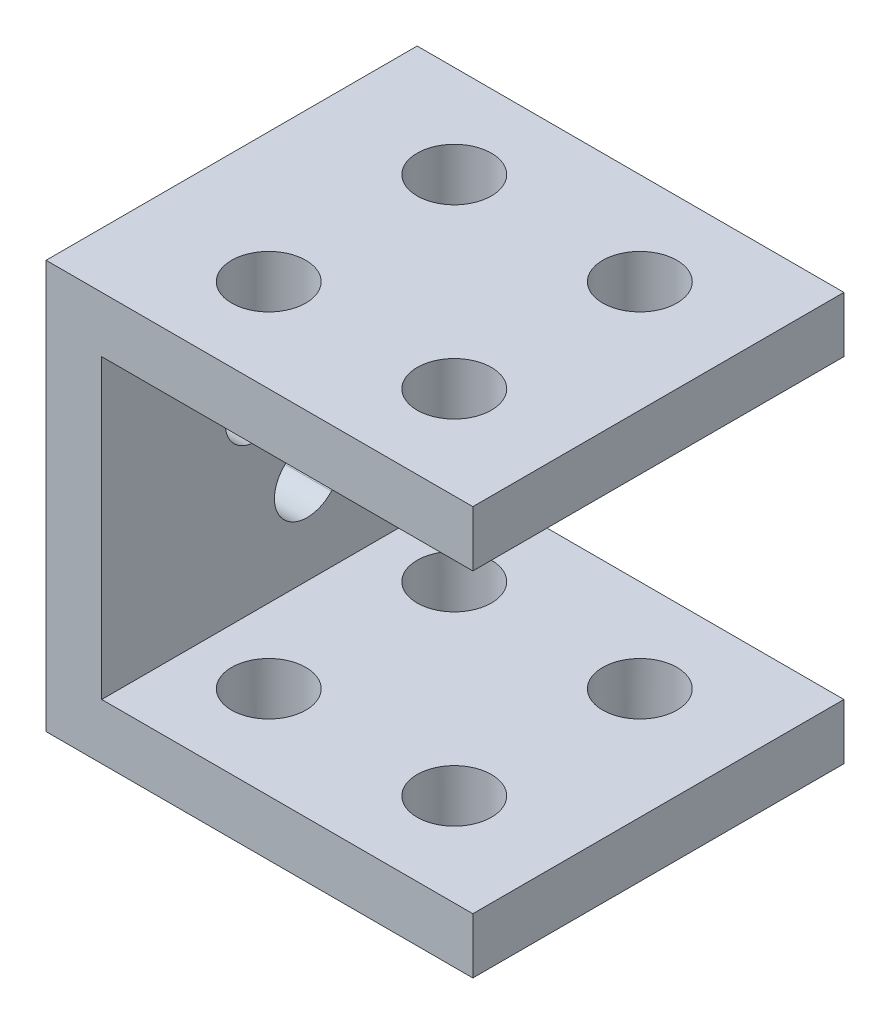
SolidWorks part; units mm, degrees
ref_plane "Front Plane" through (0, 0, 0) normal (0, 0, 1) x (1, 0, 0)
ref_plane "Top Plane" through (0, 0, 0) normal (0, 1, 0) x (1, 0, 0)
ref_plane "Right Plane" through (0, 0, 0) normal (1, 0, 0) x (0, 0, -1)
other "Configuration Table"
sketch "Sketch1" plane through (0, 0, 0) normal (0, 0, 1) x (1, 0, 0)
  line L0 (0, 0) -> (100, 0)
  line L1 (0, 0) -> (0, 80)
  line L2 (0, 80) -> (100, 80)
  line L3 (-15, -15) -> (100, -15)
  line L4 (-15, -15) -> (-15, 95)
  line L5 (-15, 95) -> (100, 95)
  line L6 (100, 95) -> (100, 80)
  line L7 (100, 0) -> (100, -15)
  dimension "D1" = 80
  dimension "D2" = 100
  dimension "D3" = 100
  dimension "D4" = 15
extrude "Boss-Extrude1" add sketch "Sketch1" along normal blind 100
sketch "Sketch2" plane through (0, 95, 0) normal (0, 1, 0) x (1, 0, 0)
  line L0 (100, -100) -> (-15, -100) construction
  line L1 (-15, -100) -> (-15, 0) construction
  line L2 (100, -100) -> (100, 0) construction
  circle A0 centre (20, -25) radius 10
  circle A1 centre (70, -25) radius 10
  circle A2 centre (20, -75) radius 10
  circle A3 centre (70, -75) radius 10
  dimension "D9" = 20
  dimension "D1" = 25
  dimension "D2" = 50
  dimension "D3" = 25
  dimension "D4" = 50
  dimension "D5" = 35
  dimension "D6" = 30
  dimension "D7" = 50
  dimension "D8" = 35
extrude "Cut-Extrude1" cut sketch "Sketch2" against normal blind 500
sketch "Sketch3" plane through (0, 0, 0) normal (1, 0, 0) x (0, 0, -1)
  line L0 (-58.6172, 47.5466) -> (-39.6015, 63.1332) construction
  line L3 (-63.7334, 53.7884) -> (-44.7177, 69.375)
  line L4 (-53.501, 41.3048) -> (-34.4852, 56.8915)
  line L11 (-44.6429, 23.5983) -> (-23.3021, 47.219) construction
  line L12 (-51.1889, 29.5125) -> (-29.8481, 53.1332)
  line L13 (-38.0969, 17.684) -> (-16.756, 41.3048)
  arc A2 (-63.7334, 53.7884) -> (-53.501, 41.3048) centre (-58.6172, 47.5466) ccw
  arc A3 (-34.4852, 56.8915) -> (-44.7177, 69.375) centre (-39.6015, 63.1332) ccw
  arc A8 (-51.1889, 29.5125) -> (-38.0969, 17.684) centre (-44.6429, 23.5983) ccw
  arc A9 (-16.756, 41.3048) -> (-29.8481, 53.1332) centre (-23.3021, 47.219) ccw
  point P2 (-49.1093, 55.3399)
  point P21 (-33.9725, 35.4086)
extrude "Cut-Extrude2" cut sketch "Sketch3" against normal blind 500
